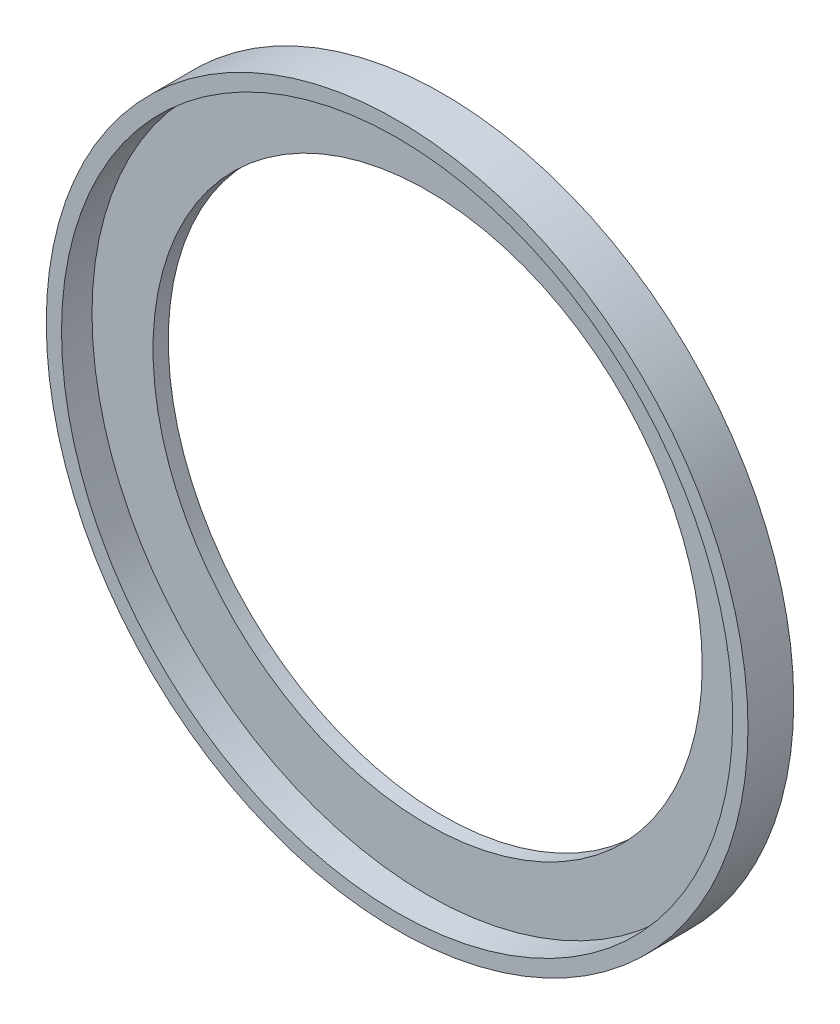
SolidWorks part; units mm, degrees
ref_plane "前视基准面" through (0, 0, 0) normal (0, 0, 1) x (1, 0, 0)
ref_plane "上视基准面" through (0, 0, 0) normal (0, 1, 0) x (1, 0, 0)
ref_plane "右视基准面" through (0, 0, 0) normal (1, 0, 0) x (0, 0, -1)
sketch "草图1" plane through (0, 0, 0) normal (0, 0, 1) x (1, 0, 0)
  circle A0 centre (0, 0) radius 105
extrude "凸台-拉伸1" add sketch "草图1" along normal blind 30
sketch "草图2" plane through (0, 0, 30) normal (0, 0, 1) x (1, 0, 0)
  circle A0 centre (0, 0) radius 90
extrude "切除-拉伸1" cut sketch "草图2" against normal blind 73
sketch "草图3" plane through (0, 0, 30) normal (0, 0, 1) x (1, 0, 0)
  circle A1 centre (0, 0) radius 90
  circle A2 centre (0, 0) radius 100
  circle A3 centre (0, 0) radius 100
  circle A4 centre (0, 0) radius 85
  circle M2 centre (0, 0) radius 90
  dimension "D1" = 5
extrude "切除-拉伸2" cut sketch "草图3" against normal blind 25 contours A3 M2
sketch "草图4" plane through (0, 0, 30) normal (0, 0, 1) x (1, 0, 0)
  circle A0 centre (0, 0) radius 110
  circle A1 centre (0, 0) radius 115
  dimension "D1" = 5
extrude "凸台-拉伸2" add sketch "草图4" against normal blind 30 separate body
sketch "草图5" plane through (0, 0, 30) normal (0, 0, 1) x (1, 0, 0)
  circle A1 centre (0, 0) radius 100
  circle A2 centre (0, 0) radius 105
  circle A3 centre (0, 0) radius 105
  dimension "D1" = 0
extrude "切除-拉伸3" cut sketch "草图5" against normal blind 25
sketch "草图6" plane through (0, 0, 0) normal (0, 0, -1) x (-1, 0, 0)
  circle A1 centre (0, 0) radius 110
  circle A2 centre (0, 0) radius 105
  circle A3 centre (0, 0) radius 105
  dimension "D1" = 0
  dimension "D2" = 5
extrude "凸台-拉伸3" add sketch "草图6" against normal blind 5
sketch "草图7" plane through (0, 0, 30) normal (0, 0, 1) x (1, 0, 0)
  circle A2 centre (0, 0) radius 125
  circle A3 centre (0, 0) radius 125
  dimension "D1" = 10
extrude "切除-拉伸5" cut sketch "草图7" against normal blind 15
